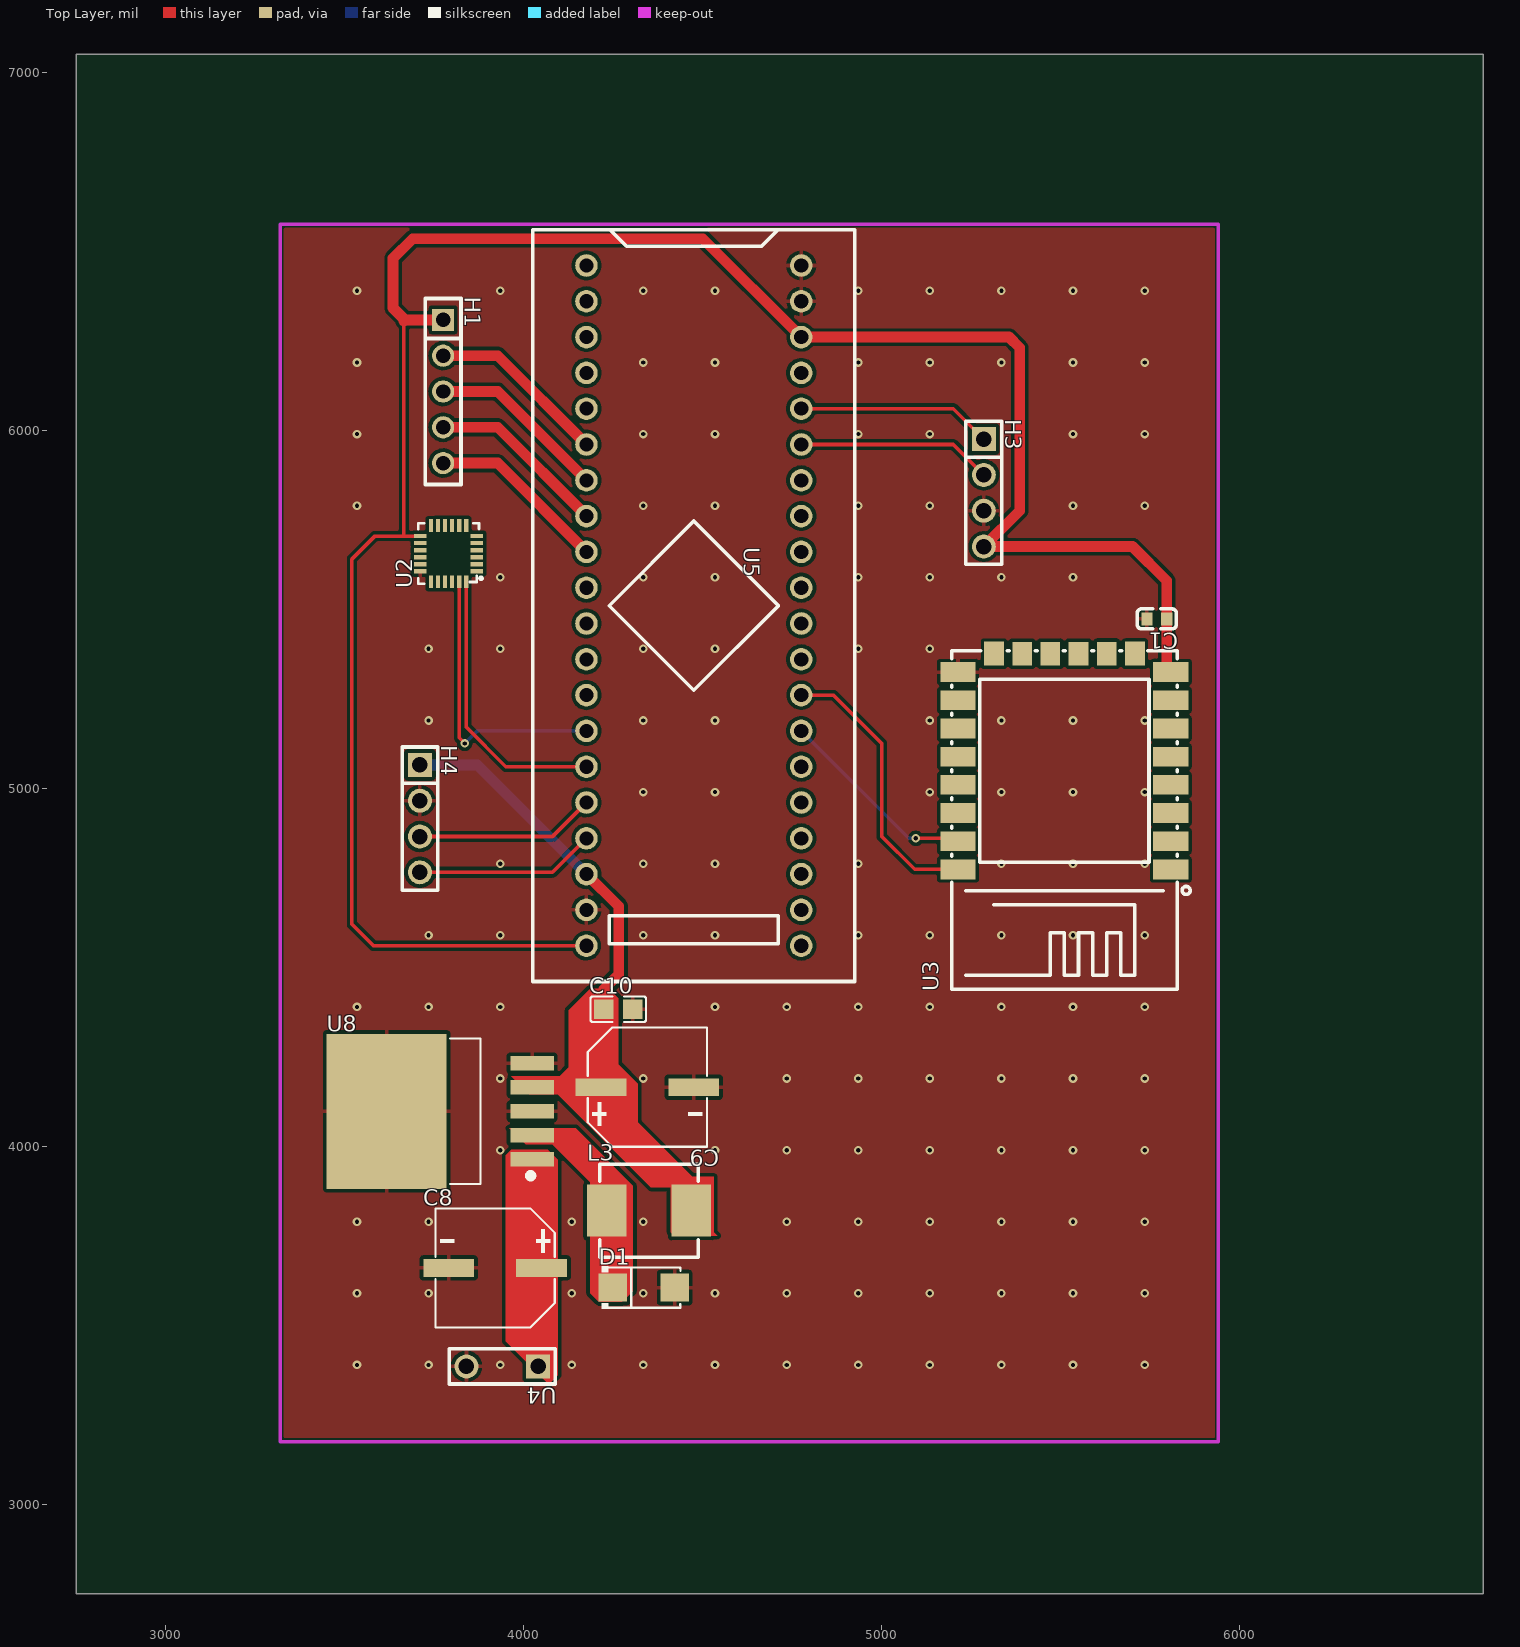
[diagram p0: Top Layer view]
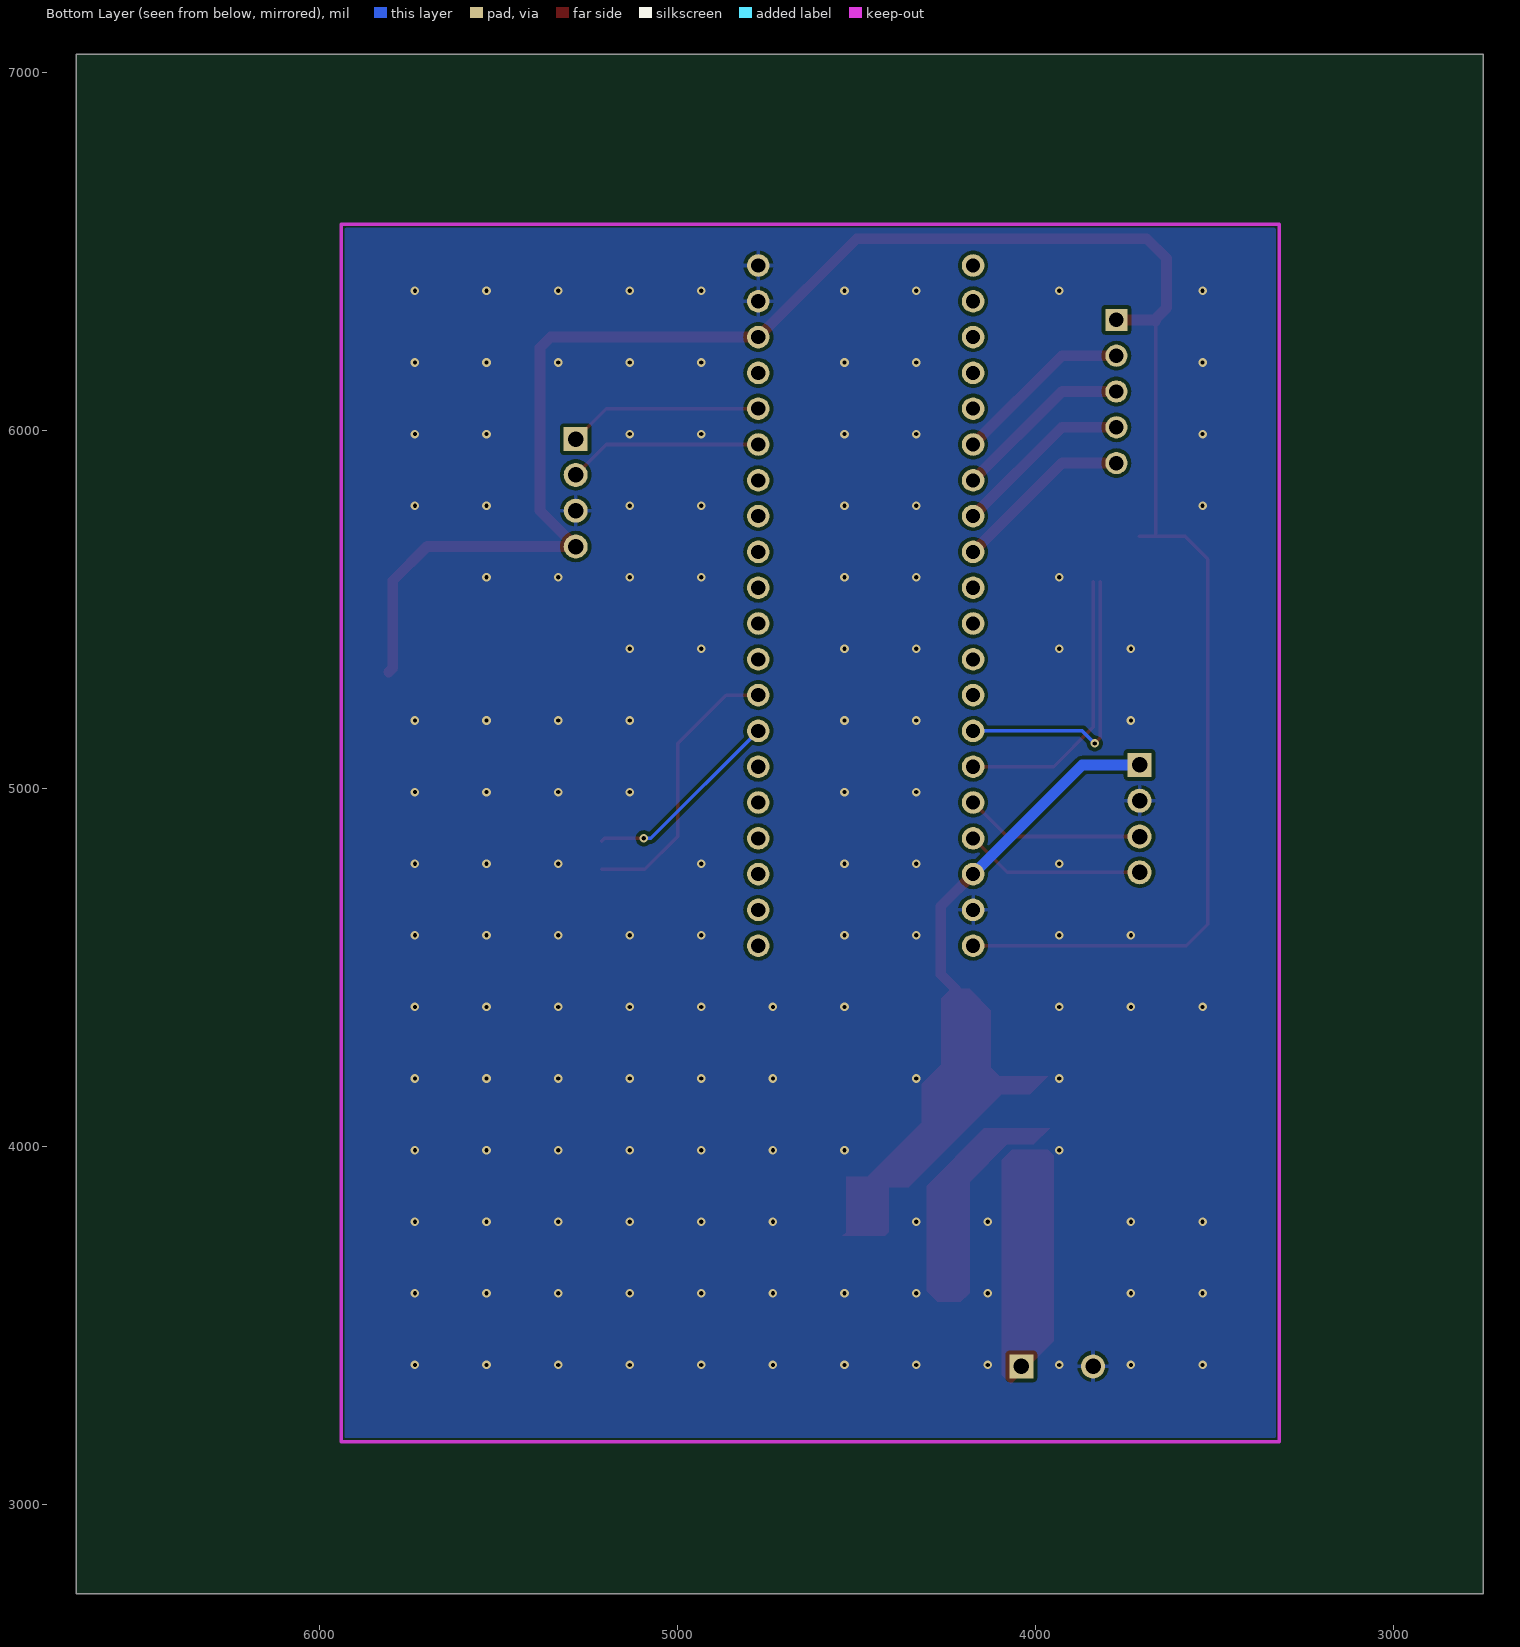
[diagram p1: Bottom Layer view, seen from below]
# Altium PCB MISC52071.pcbdoc
Units mil, origin at the board's own origin, x right, y up, seen from the top; angles counter-clockwise.
Board outline 3930 x 4300 mil, 2 copper layers (Top Layer, Bottom Layer), stack 62.206 mil thick; 14 components, 17 nets, 119 pads, 134 vias.

## Layer stack, top to bottom
Top Solder Mask Layer: solder mask 0.394, Dk 3.3
Top Layer: signal copper 1.379
Dielectric1: surface 59.449, FR4, Dk 4.5
Bottom Layer: signal copper 1.378
Bottom Solder Mask Layer: solder mask 0.394, Dk 3.3

## Board outline
6680,2750 2750,2750 2750,7050 6680,7050

## Design rules (kind name [scope] priority, off if disabled: settings)
BoardOutlineClearance copperThickness2oz_1 [All] p2 off: genericclearance=7.99 ignorepadtopadclearanceinfootprint=FALSE except(0: Arc-SplitContinuation Track-SplitContinuation SMDPad-SplitContinuation THPad-SplitContinuation Via-SplitContinuation Fill-SplitContinuation Region-SplitContinuation Poly-SplitContinuation Text-SplitContinuation Hole-SplitContinuation; 5.98: Arc-CutoutEdge SMDPad-CutoutEdge THPad-CutoutEdge Via-CutoutEdge Fill-CutoutEdge Region-CutoutEdge Text-CutoutEdge; 6.93: Hole-OutlineEdge Hole-CutoutEdge; 10: Poly-OutlineEdge Poly-CutoutEdge; 11.81: Arc-OutlineEdge Track-OutlineEdge SMDPad-OutlineEdge THPad-OutlineEdge Via-OutlineEdge Fill-OutlineEdge Region-OutlineEdge Text-OutlineEdge Track-CutoutEdge)
BoardOutlineClearance copperThickness1oz_1 [All] p4: genericclearance=4.02 ignorepadtopadclearanceinfootprint=FALSE except(0: Arc-SplitContinuation Track-SplitContinuation SMDPad-SplitContinuation THPad-SplitContinuation Via-SplitContinuation Fill-SplitContinuation Region-SplitContinuation Poly-SplitContinuation Text-SplitContinuation Hole-SplitContinuation; 6: SMDPad-CutoutEdge THPad-CutoutEdge Via-CutoutEdge Fill-CutoutEdge Region-CutoutEdge Text-CutoutEdge; 6.93: Hole-OutlineEdge Hole-CutoutEdge; 10: Poly-OutlineEdge Poly-CutoutEdge; 11.8: Arc-OutlineEdge Track-OutlineEdge SMDPad-OutlineEdge THPad-OutlineEdge Via-OutlineEdge Fill-OutlineEdge Region-OutlineEdge Text-OutlineEdge; 11.81: Arc-CutoutEdge Track-CutoutEdge)
Clearance copperThickness2oz [All] p1 off: gap=7.99 ignorepadtopadclearanceinfootprint=FALSE except(5.98: SMDPad-Track SMDPad-SMDPad THPad-Track SMDPad-THPad THPad-THPad Track-Via SMDPad-Via THPad-Via Via-Via Fill-Track Region-Track Fill-SMDPad Region-SMDPad Fill-THPad Region-THPad Fill-Via Region-Via Fill-Fill Fill-Region Region-Region Arc-Track Arc-SMDPad Arc-THPad Arc-Via Fill-Arc Region-Arc Arc-Arc Text-Track SMDPad-Text Text-THPad Text-Via Fill-Text Region-Text Arc-Text Text-Text; 6.93: Hole-Track Hole-SMDPad Hole-THPad Hole-Via Fill-Hole Region-Hole Hole-Arc Hole-Text; 10: Poly-Track Poly-SMDPad Poly-THPad Poly-Via Poly-Fill Poly-Region Poly-Poly Poly-Arc Poly-Text Poly-Hole)
Clearance copperThickness1oz [All] p3: gap=4.02 ignorepadtopadclearanceinfootprint=FALSE except(5.98: SMDPad-Track SMDPad-SMDPad THPad-Track SMDPad-THPad THPad-THPad Track-Via SMDPad-Via THPad-Via Via-Via Fill-Track Region-Track Fill-SMDPad Region-SMDPad Fill-THPad Region-THPad Fill-Via Region-Via Fill-Fill Fill-Region Region-Region; 6: Arc-Track Arc-SMDPad Arc-THPad Arc-Via Fill-Arc Region-Arc Arc-Arc Text-Track SMDPad-Text Text-THPad Text-Via Fill-Text Region-Text Arc-Text Text-Text; 6.93: Hole-Track Hole-SMDPad Hole-THPad Hole-Via Fill-Hole Region-Hole Hole-Arc Hole-Text; 10: Poly-Track Poly-SMDPad Poly-THPad Poly-Via Poly-Fill Poly-Region Poly-Poly Poly-Arc Poly-Text Poly-Hole)
DiffPairsRouting differentialPair [All] p1: maxlimit=6 minlimit=6 mostfreqgap=6 toplayer_minwidth=5 toplayer_prefwidth=10 toplayer_maxwidth=100 toplayer_mingap=6 toplayer_prefgap=6 toplayer_maxgap=6 bottomlayer_minwidth=5 bottomlayer_prefwidth=10 bottomlayer_maxwidth=100 bottomlayer_mingap=6 bottomlayer_prefgap=6 bottomlayer_maxgap=6 maxuncoupledlength=10
HoleToHoleClearance otherClearance [All] p1: gap=11.81 allowstackedmicrovias=TRUE
Length netLength [All] p1: minlimit=0 maxlimit=0
MatchedLengths netLengthTolerance [All] p1: tolerance=1000
PasteMaskExpansion pasteMaskExpansion [All] p1: expansion=0
PlaneConnect innerPlane [All] p1: planeconnectstyle=Relief reliefexpansion=20 reliefentries=4 reliefconductorwidth=10 reliefairgap=10
PolygonConnect copperRegion [(InNet('GND'))] p1: connectstyle=Relief reliefconductorwidth=10 reliefentries=4 polygonreliefangle="90 Angle" airgapwidth=10 via.connectstyle=Relief via.reliefconductorwidth=10 via.reliefentries=4 via.polygonreliefangle="90 Angle" via.airgapwidth=10
RoutingVias viaSize [All] p1: holewidth=12.01 width=24.02 viastyle="Through Hole" minholewidth=11.81 minwidth=19.68 maxholewidth=248.03 maxwidth=393.7
SolderMaskExpansion solderMaskExpansion [IsVia] p1: expansion=-1000 istentingtop=TRUE
SolderMaskExpansion solderMaskExpansion [All] p2: expansion=2 istentingtop=FALSE
Width copperThickness2oz_2 [All] p1 off: maxlimit=100 minlimit=8 preferedwidth=10
Width copperThickness1oz_2 [All] p2: maxlimit=100 minlimit=5 preferedwidth=10

## Components (designator, comment, footprint, x,y, rotation, side; value= is the part's Value field where it differs from the comment)
C1 "10uF" C0603 5768.16,5472.84 r180 top
C8 "" CAP-SMD_BD8.0-L8.3-W8.3-RD 3920,3660 r0 top
C9 "" CAP-SMD_BD8.0-L8.3-W8.3-RD 4345,4165 r180 top
C10 "" C0805 4263.85,4382.57 r0 top
D1 "" SMA_L4.3-W2.6-LS5.2-RD 4335,3605 r0 top
H1 "" HDR-TH_5P-P2.54-V-F 3774.74,6108.05 r270 top
H3 "Encoder" HDR-TH_4P-P2.54-V-M 5285,5825 r270 top
H4 "Servo" HDR-TH_4P-P2.54-V-M 3710,4915 r270 top
L3 "" IND-SMD_L7.0-W6.6 4350,3820 r0 top
U2 "MPU6050" QFN-24_L4.0-W4.0-P0.50-BL 3790,5655 r90 top
U3 "ESP8266" WIFIM-SMD_ESP-12F-ESP8266MOD 5510.06,5074.4 r90 top
U4 "5.08-2PIN straight header" HDR-TH_2P-P5.08_C9900004333 3940,3385 r180 top
U5 "STM32F103C8T6-Card" CONN-TH_L53.3-W22.9_STM32F103C8T6-CARD 4475,5510 r270 top
U8 "LM2596S-5.0" TO-263-5_L10.2-W8.9-P1.70-BR 3820.03,4097.57 r0 top

## Footprints (in the part's own frame and the unit in brackets; to place one, negate y for a bottom-side part, rotate by r counter-clockwise, add the part's x,y. Pads: shape width x height; smd on the part's side, far side on the other; paste and mask are expansions set on the pad)
C0603 [mm]
  rect 0.8x0.9 smd: 1(-0.7,0) 2(0.7,0)
  silkscreen extent -1.39,-0.71 1.39,0.71
C0805 [mm]
  rect 1.41x1.35 smd paste-100 mask+0.051: 1(-1.03,0) 2(1.03,0)
  silkscreen extent -1.96,-0.9 1.96,0.9
CAP-SMD_BD8.0-L8.3-W8.3-RD [mm]
  rect 3.61x1.26 smd paste+0 mask+0.051: 1(3.295,0) 2(-3.295,0)
  silkscreen extent -4.23,-4.23 4.23,4.23
CONN-TH_L53.3-W22.9_STM32F103C8T6-CARD [mm]
  round 1.6 hole 1: 1(-24.13,-7.62) 2(-21.59,-7.62) 3(-19.05,-7.62) 4(-16.51,-7.62) 5(-13.97,-7.62) 6(-11.43,-7.62) 7(-8.89,-7.62) 8(-6.35,-7.62) 9(-3.81,-7.62) 10(-1.27,-7.62) 11(1.27,-7.62) 12(3.81,-7.62) 13(6.35,-7.62) 14(8.89,-7.62) 15(11.43,-7.62) 16(13.97,-7.62) 17(16.51,-7.62) 18(19.05,-7.62) 19(21.59,-7.62) 20(24.13,-7.62) 21(24.13,7.62) 22(21.59,7.62) 23(19.05,7.62) 24(16.51,7.62) 25(13.97,7.62) 26(11.43,7.62) 27(8.89,7.62) 28(6.35,7.62) 29(3.81,7.62) 30(1.27,7.62) 31(-1.27,7.62) 32(-3.81,7.62) 33(-6.35,7.62) 34(-8.89,7.62) 35(-11.43,7.62) 36(-13.97,7.62) 37(-16.51,7.62) 38(-19.05,7.62) 39(-21.59,7.62) 40(-24.13,7.62)
  silkscreen extent -26.67,-11.43 26.67,11.43
HDR-TH_2P-P5.08_C9900004333 [mm]
  rect 1.7x1.7 hole 1.1 paste+0 mask+0.05: 1(-2.54,0)
  round 1.7 hole 1.1 paste+0 mask+0.05: 2(2.54,0)
  silkscreen extent -3.75,-1.25 3.75,1.25
HDR-TH_4P-P2.54-V-M [mm]
  rect 1.7x1.7 hole 1.1: 1(-3.81,0)
  round 1.7 hole 1.1: 2(-1.27,0) 3(1.27,0) 4(3.81,0)
  silkscreen extent -5.08,-1.27 5.08,1.27
HDR-TH_5P-P2.54-V-F [mil]
  rect 62x62 hole 40.16: 1(-200,0)
  round 62 hole 40.16: 2(-100,0) 3(0,0) 4(100,0) 5(200,0)
  silkscreen extent -260,-50 260,50
IND-SMD_L7.0-W6.6 [mil]
  rect 110.2x145.7 smd paste+0 mask+2: 1(-118.1,0) 2(118.1,0)
  silkscreen extent -138,-130 138,130
QFN-24_L4.0-W4.0-P0.50-BL [mm]
  rect 0.3x0.9 smd paste+0 mask+0.05: 1(-1.25,-2) 2(-0.75,-2) 3(-0.25,-2) 4(0.25,-2) 5(0.75,-2) 6(1.25,-2) 13(1.25,2) 14(0.75,2) 15(0.25,2) 16(-0.25,2) 17(-0.75,2) 18(-1.25,2)
  rect 0.9x0.3 smd paste+0 mask+0.05: 7(2,-1.25) 8(2,-0.75) 9(2,-0.25) 10(2,0.25) 11(2,0.75) 12(2,1.25) 19(-2,1.25) 20(-2,0.75) 21(-2,0.25) 22(-2,-0.25) 23(-2,-0.75) 24(-2,-1.25)
  silkscreen extent -2.14,-2.4 2.16,2.15
SMA_L4.3-W2.6-LS5.2-RD [mm]
  rect 2x2 smd paste+0 mask+0.051: 1(-2.2,0) 2(2.2,0)
  silkscreen extent -2.98,-1.5 2.6,1.5
TO-263-5_L10.2-W8.9-P1.70-BR [mm]
  rect 3.083x1.02 smd: 1(5.16,-3.4) 2(5.16,-1.7) 3(5.16,0) 4(5.16,1.7) 5(5.16,3.4)
  rect 8.5x11 smd: 6(-5.16,0)
  silkscreen extent -0.66,-5.16 5.26,5.16
WIFIM-SMD_ESP-12F-ESP8266MOD [mm]
  rect 1.4x2.5 smd: 1(-7.651,-7.551) 2(-5.651,-7.551) 3(-3.651,-7.551) 4(-1.651,-7.551) 5(0.349,-7.551) 6(2.349,-7.551) 7(4.349,-7.551) 8(6.349,-7.551) 9(6.349,7.549) 10(4.349,7.55) 11(2.349,7.551) 12(0.349,7.551) 13(-1.651,7.55) 14(-3.651,7.551) 15(-5.651,7.55) 16(-7.651,7.551)
  rect 1.7x1.4 smd: 17(7.651,-5) 18(7.649,-3.002) 19(7.65,-1.003) 20(7.65,0.997) 21(7.65,2.997) 22(7.65,4.997)
  silkscreen extent -16.15,-8.92 7.85,8

## Via types
v1: diameter 24.02, hole 12, Top Layer to Bottom Layer, 134 vias

## Nets (pads, with @x,y where several pads share a name; then routed paths per layer and width w, separated by ;. In a path a pad name is that pad's centre, name@x,y a point inside that pad or via, vN(x,y) a via of type N, cw(c..) or ccw(c..) an arc to the next point about the centre after c; other vN are vias at no path point)
3.3V: C1.1 H1.1 H3.4 U2.13 U3.8 U5.20 U5.38 | length 6120.6
  Top Layer w10: 3665.27,6305 3665.27,5704.21 ; U2.13 3665.27,5704.21 ; U5.20 3580,4560 3520,4620 3520,5640 3584.21,5704.21 3665.27,5704.21
  Top Layer w30: 3665.27,6305 3668.32,6308.05 ; H1.1 3668.32,6308.05 ; U3.8 5795.72,5335.98 C1.1 5795.72,5579.28 5700,5675 H3.4 5385,5775 5385,6230 5355,6260 U5.38 4500,6535 3690,6535 3635,6480 3635,6341.37 3668.32,6308.05
5VOUT: C9.1 C10.1 H4.1 L3.2 U5.18 U8.4 | length 1023.3
  Top Layer w30: U5.18 4265,4670 4265,4480 4223.3,4438.3 C10.1
  Bottom Layer w30: H4.1 3870,5065 U5.18
12V: C8.1 U4.1 U8.1
$1N90: D1.1 L3.1 U8.2
$1N99: H4.4 U5.17 | length 504.4
  Top Layer w10: H4.4 4080,4765 U5.17
$1N100: H4.3 U5.16 | length 504.4
  Top Layer w10: H4.3 4080,4865 U5.16
$1N108: H3.2 U5.35 | length 545.2
  Top Layer w10: U5.35 5200,5960 H3.2
$1N109: H3.1 U5.36 | length 545.2
  Top Layer w10: U5.36 5200,6060 H3.1
$1N113: H1.2 U5.6 | length 503
  Top Layer w30: H1.2 3926.95,6208.05 U5.6
$1N114: H1.3 U5.7 | length 503
  Top Layer w30: H1.3 3926.95,6108.05 U5.7
$1N115: H1.4 U5.8 | length 503
  Top Layer w30: H1.4 3926.95,6008.05 U5.8
$1N116: H1.5 U5.9 | length 503
  Top Layer w30: H1.5 3926.95,5908.05 U5.9
GND: C1.2 C8.2 C9.2 C10.2 D1.2 H3.3 H4.2 U2.18 U3.9 U4.2 U5.19 U5.39 U5.40 U8.3 U8.5 U8.6
  other v1: 3534.1,3389.1 3734.1,3389.1 3934.1,3389.1 4134.1,3389.1 4334.1,3389.1 4534.1,3389.1 4734.1,3389.1 4934.1,3389.1 5134.1,3389.1 5334.1,3389.1 5534.1,3389.1 5734.1,3389.1 3534.1,3589.1 3734.1,3589.1 4134.1,3589.1 4334.1,3589.1 4534.1,3589.1 4734.1,3589.1 4934.1,3589.1 5134.1,3589.1 5334.1,3589.1 5534.1,3589.1 5734.1,3589.1 3534.1,3789.1 3734.1,3789.1 4134.1,3789.1 4334.1,3789.1 4734.1,3789.1 4934.1,3789.1 5134.1,3789.1 5334.1,3789.1 5534.1,3789.1 5734.1,3789.1 3934.1,3989.1 4534.1,3989.1 4734.1,3989.1 4934.1,3989.1 5134.1,3989.1 5334.1,3989.1 5534.1,3989.1 5734.1,3989.1 3934.1,4189.1 4334.1,4189.1 4734.1,4189.1 4934.1,4189.1 5134.1,4189.1 5334.1,4189.1 5534.1,4189.1 5734.1,4189.1 3534.1,4389.1 3734.1,4389.1 3934.1,4389.1 4534.1,4389.1 4734.1,4389.1 4934.1,4389.1 5134.1,4389.1 5334.1,4389.1 5534.1,4389.1 5734.1,4389.1 3734.1,4589.1 3934.1,4589.1 4334.1,4589.1 4534.1,4589.1 4934.1,4589.1 5134.1,4589.1 5334.1,4589.1 5534.1,4589.1 5734.1,4589.1 3934.1,4789.1 4334.1,4789.1 4534.1,4789.1 4934.1,4789.1 5334.1,4789.1 5534.1,4789.1 5734.1,4789.1 4334.1,4989.1 4534.1,4989.1 5134.1,4989.1 5334.1,4989.1 5534.1,4989.1 5734.1,4989.1 3734.1,5189.1 4334.1,5189.1 4534.1,5189.1 5134.1,5189.1 5334.1,5189.1 5534.1,5189.1 5734.1,5189.1 3734.1,5389.1 3934.1,5389.1 4334.1,5389.1 4534.1,5389.1 4934.1,5389.1 5134.1,5389.1 3934.1,5589.1 4334.1,5589.1 4534.1,5589.1 4934.1,5589.1 5134.1,5589.1 5334.1,5589.1 5534.1,5589.1 3534.1,5789.1 4334.1,5789.1 4534.1,5789.1 4934.1,5789.1 5134.1,5789.1 5534.1,5789.1 5734.1,5789.1 3534.1,5989.1 4334.1,5989.1 4534.1,5989.1 4934.1,5989.1 5134.1,5989.1 5534.1,5989.1 5734.1,5989.1 3534.1,6189.1 4334.1,6189.1 4534.1,6189.1 4934.1,6189.1 5134.1,6189.1 5334.1,6189.1 5534.1,6189.1 5734.1,6189.1 3534.1,6389.1 3934.1,6389.1 4334.1,6389.1 4534.1,6389.1 4934.1,6389.1 5134.1,6389.1 5334.1,6389.1 5534.1,6389.1 5734.1,6389.1
MPU60501: U2.23 U5.14 | length 812.2
  Top Layer w10: U2.23 3819.53,5140.47 v1(3835,5125)
  Bottom Layer w10: v1(3835,5125) 3870,5160 U5.14
MPU60502: U2.24 U5.15 | length 787.2
  Top Layer w10: U2.24 3839.21,5170.79 3950,5060 U5.15
RXD: U3.15 U5.27 | length 565.4
  Top Layer w10: v1(5095,4860) 5204.73,4860 U3.15
  Bottom Layer w10: U5.27 5075,4860 v1(5095,4860)
TXD: U3.16 U5.28 | length 791.7
  Top Layer w10: U5.28 4865,5260 5000,5125 5000,4865 5091.8,4773.2 U3.16
pads on no net: U2.1 U2.2 U2.3 U2.4 U2.5 U2.6 U2.7 U2.8 U2.9 U2.10 U2.11 U2.12 U2.14 U2.15 U2.16 U2.17 U2.19 U2.20 U2.21 U2.22 U3.1 U3.2 U3.3 U3.4 U3.5 U3.6 U3.7 U3.10 U3.11 U3.12 U3.13 U3.14 U3.17 U3.18 U3.19 U3.20 U3.21 U3.22 U5.1 U5.2 U5.3 U5.4 U5.5 U5.10 U5.11 U5.12 U5.13 U5.21 U5.22 U5.23 U5.24 U5.25 U5.26 U5.29 U5.30 U5.31 U5.32 U5.33 U5.34 U5.37

## Polygon pours and split planes (outlines as drawn)
GND on Top Layer (solid, remove dead copper, pour order 0): 3000,6800 3000,3000 6430,3000 6430,6800
GND on Bottom Layer (solid, remove dead copper, pour order 2): 3180,6730 3180,3080 6320,3080 6320,6730

## Keep-outs
Board Outline Layer:
  lines w10: 3320,3175 3320,6575 5940,6575 5940,3175 3320,3175

## Other copper
Top Layer:
  region net 5VOUT: 3965,4195 4100,4195 4125,4220 4125,4380 4185,4440 4237.76,4440 4263.85,4413.91 4263.85,4229.62 4318.46,4175 4318.46,4066.54 4470,3915 4530,3915 4530,3760 4540,3750 4420,3750 4410,3760 4410,3885 4355,3885 4095,4145 4015,4145
  region net $1N90: 3960,4050 4145,4050 4305,3890 4305,3595 4275,3565 4210,3565 4185,3590 4185,3900 4080,4005 4005,4005
  region net 12V: 3965,3990 4067.13,3990 4094.56,3962.57 4094.56,3360.81 4069.54,3335.79 4069.21,3335.79 3950,3455 3950,3975